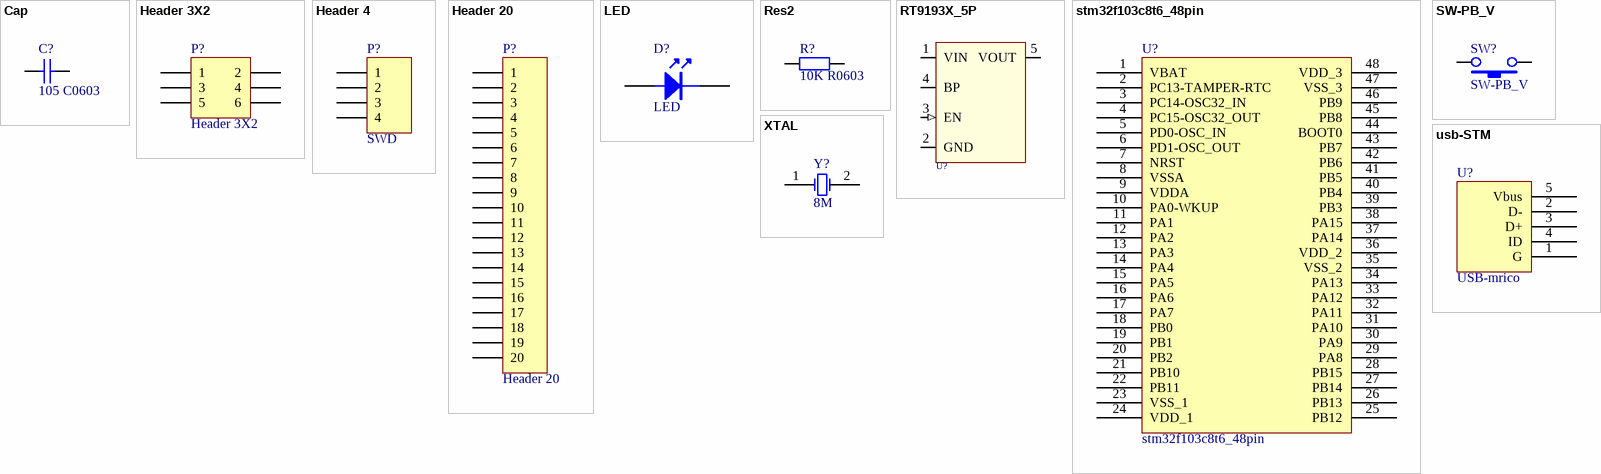
[diagram p0: symbols Cap to XTAL]
# Altium schematic symbol library MISC82227-3.SchLib: 11 symbols
Pins are listed as number, name and electrical type; pins without a type are passive.


## Cap
designator C?, comment 105 C0603
Value: 104
simulation model CAP (Capacitor)
signal-integrity model Cap
footprint C 0603 (Non-polarised SMD capacitor)
pins: 1, 2

## Header 3X2
designator P?
Header, 3-Pin, Dual row
signal-integrity model Connector
footprint HDR-3X2 (Dual-row pin header, 3x2 pins)
pins: 1, 2, 3, 4, 5, 6

## Header 4
designator P?, comment SWD
Header, 4-Pin
signal-integrity model Connector
footprint HDR-1X4_H (Right-angle pin header, 4 pins)
pins: 1, 2, 3, 4

## Header 20
designator P?
Header, 20-Pin
signal-integrity model Connector
footprint HDR1X20 (Connector; Header; 20 Position)
pins: 1, 2, 3, 4, 5, 6, 7, 8, 9, 10, 11, 12, 13, 14, 15, 16, 17, 18, 19, 20

## LED
designator D?
footprint LED 0805G (Green 0805LED)
pins: 1, 2

## Res2
designator R?, comment 10K R0603
simulation model RESISTOR (Resistor)
signal-integrity model Res
footprint R 0603 (1/10W SMD resistor)
pins: 1, 2

## RT9193X_5P
designator U?, comment RT9193  (value not drawn)
ICA_MFR_NAME: RICHTEK; ICA_PARTNUM: $$2191094$$RT9193-15CU5; Part Number: TMP-13
footprint SOT23-5L (3x1.6x1.1mm (LxWxH))
pins: 1 VIN (power), 2 GND (power), 3 EN (in), 4 BP, 5 VOUT (power)

## stm32f103c8t6_48pin
designator U?
footprint TQFP48 7x7_L (48 pins, body: 7x7mm, pitch: 0.5mm)
footprint TQFP48 7x7_L (48 pins, body: 7x7mm, pitch: 0.5mm)
pins: 1 VBAT, 2 PC13-TAMPER-RTC, 3 PC14-OSC32_IN, 4 PC15-OSC32_OUT, 5 PD0-OSC_IN, 6 PD1-OSC_OUT, 7 NRST, 8 VSSA, 9 VDDA, 10 PA0-WKUP, 11 PA1, 12 PA2, 13 PA3, 14 PA4, 15 PA5, 16 PA6, 17 PA7, 18 PB0, 19 PB1, 20 PB2, 21 PB10, 22 PB11, 23 VSS_1, 24 VDD_1, 25 PB12, 26 PB13, 27 PB14, 28 PB15, 29 PA8, 30 PA9, 31 PA10, 32 PA11, 33 PA12, 34 PA13, 35 VSS_2, 36 VDD_2, 37 PA14, 38 PA15, 39 PB3, 40 PB4, 41 PB5, 42 PB6, 43 PB7, 44 BOOT0, 45 PB8, 46 PB9, 47 VSS_3, 48 VDD_3

## SW-PB_V
designator SW?
footprint TSW SMD-3*6*2.5 (3*6*2.5mm)
pins: 1, 2

## usb-STM
designator U?, comment USB-mrico
footprint USB-micro_B (Micro USB, 5.7*7.8*2.5mm)
footprint USB-micro_B (Micro USB, 5.7*7.8*2.5mm)
pins: 1 G, 2 D-, 3 D+, 4 ID, 5 Vbus

## XTAL
designator Y?, comment 8M
Crystal Oscillator
simulation model XTAL (Spice Subcircuit)
footprint XTAL-49S DIP
footprint XTAL-49S DIP
pins: 1 OSC1, 2 OSC2